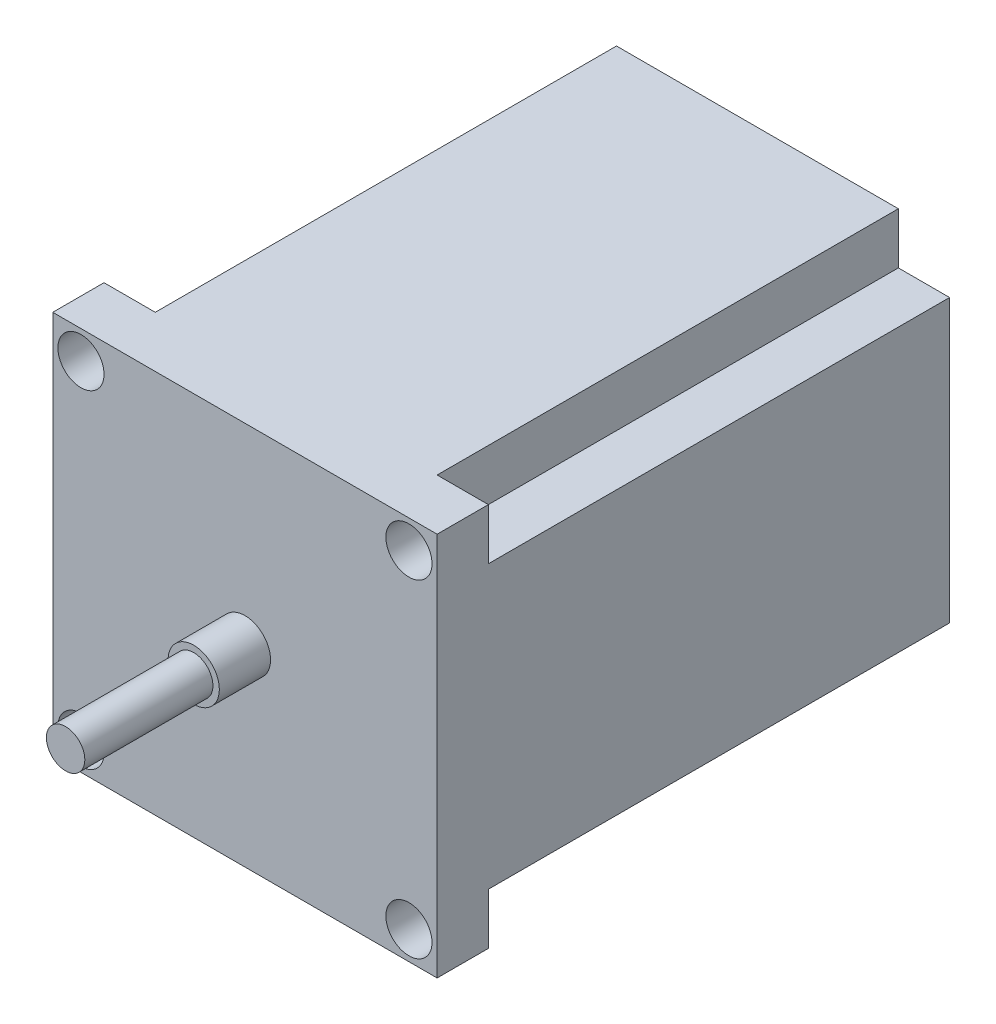
SolidWorks part; units mm, degrees
ref_plane "Front Plane" through (0, 0, 0) normal (0, 0, 1) x (1, 0, 0)
ref_plane "Top Plane" through (0, 0, 0) normal (0, 1, 0) x (1, 0, 0)
ref_plane "Right Plane" through (0, 0, 0) normal (1, 0, 0) x (0, 0, -1)
sketch "Sketch1" plane through (0, 0, 0) normal (0, 0, 1) x (1, 0, 0)
  line L1 (-7.5, -7.5) -> (7.5, -7.5)
  line L2 (-7.5, -7.5) -> (-7.5, 7.5)
  line L3 (-7.5, 7.5) -> (7.5, 7.5)
  line L4 (7.5, -7.5) -> (7.5, 7.5)
  line L5 (-7.5, -7.5) -> (7.5, 7.5) construction
  line L6 (-7.5, 7.5) -> (7.5, -7.5) construction
  point P0 (0, 0)
  dimension "D1" = 15
  dimension "D2" = 15
extrude "Boss-Extrude1" add sketch "Sketch1" along normal blind 20
sketch "Sketch2" plane through (0, 0, 20) normal (0, 0, 1) x (1, 0, 0)
  circle A0 centre (0, 0) radius 9.051 construction
  circle A1 centre (6.4, 6.4) radius 0.9
  circle A2 centre (-6.4, 6.4) radius 0.9
  circle A3 centre (-6.4, -6.4) radius 0.9
  circle A4 centre (6.4, -6.4) radius 0.9
  dimension "D3" = 1.8
  dimension "D5" = 1.8
  dimension "D6" = 1.8
  dimension "D1" = 12.8
  dimension "D2" = 12.8
sketch "Sketch5" plane through (0, 0, 0) normal (0, 0, -1) x (-1, 0, 0)
  line L1 (7.5, 7.5) -> (5.5, 7.5)
  line L2 (7.5, 7.5) -> (7.5, 5.5)
  line L3 (7.5, 5.5) -> (5.5, 5.5)
  line L4 (5.5, 7.5) -> (5.5, 5.5)
  line L5 (7.5, -7.5) -> (5.5, -7.5)
  line L6 (7.5, -7.5) -> (7.5, -5.5)
  line L7 (7.5, -5.5) -> (5.5, -5.5)
  line L8 (5.5, -7.5) -> (5.5, -5.5)
  line L9 (-7.5, -7.5) -> (-5.5, -7.5)
  line L10 (-7.5, -7.5) -> (-7.5, -5.5)
  line L11 (-7.5, -5.5) -> (-5.5, -5.5)
  line L12 (-5.5, -7.5) -> (-5.5, -5.5)
  line L13 (-7.5, 7.5) -> (-5.5, 7.5)
  line L14 (-7.5, 7.5) -> (-7.5, 5.5)
  line L15 (-7.5, 5.5) -> (-5.5, 5.5)
  line L16 (-5.5, 7.5) -> (-5.5, 5.5)
  dimension "D1" = 2
  dimension "D2" = 2
  dimension "D3" = 2
  dimension "D4" = 2
  dimension "D5" = 2
  dimension "D6" = 2
  dimension "D7" = 2
  dimension "D8" = 2
extrude "Cut-Extrude1" cut sketch "Sketch5" against normal blind 18
extrude "Cut-Extrude2" cut sketch "Sketch2" against normal blind 71
sketch "Sketch6" plane through (0, 0, 20) normal (0, 0, 1) x (1, 0, 0)
  circle A0 centre (0, 0) radius 1
  dimension "D1" = 2
extrude "Boss-Extrude2" add sketch "Sketch6" along normal blind 2
sketch "Sketch7" plane through (0, 0, 22) normal (0, 0, 1) x (1, 0, 0)
  circle A0 centre (0, 0) radius 0.75
  dimension "D1" = 1.5
extrude "Boss-Extrude3" add sketch "Sketch7" along normal blind 5
